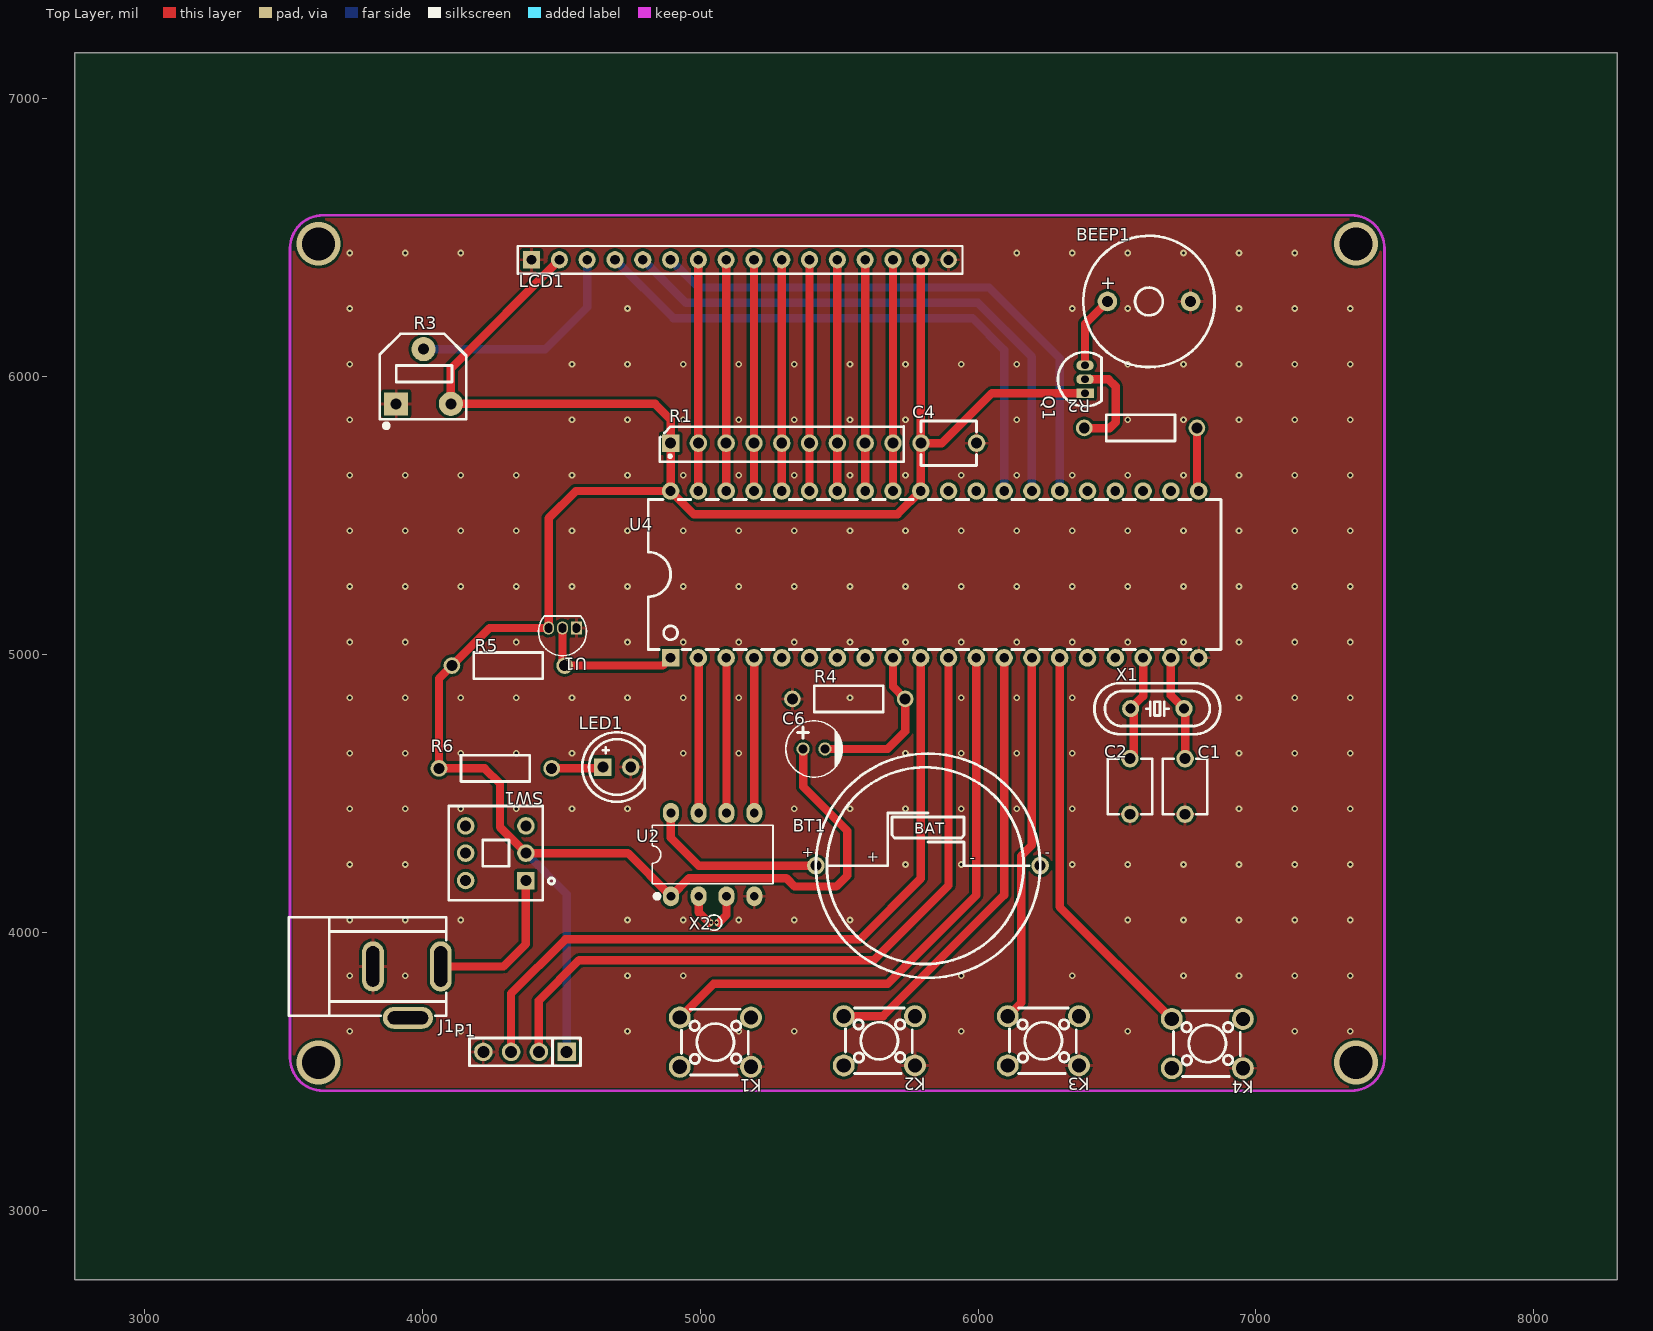
[diagram p0: Top Layer view]
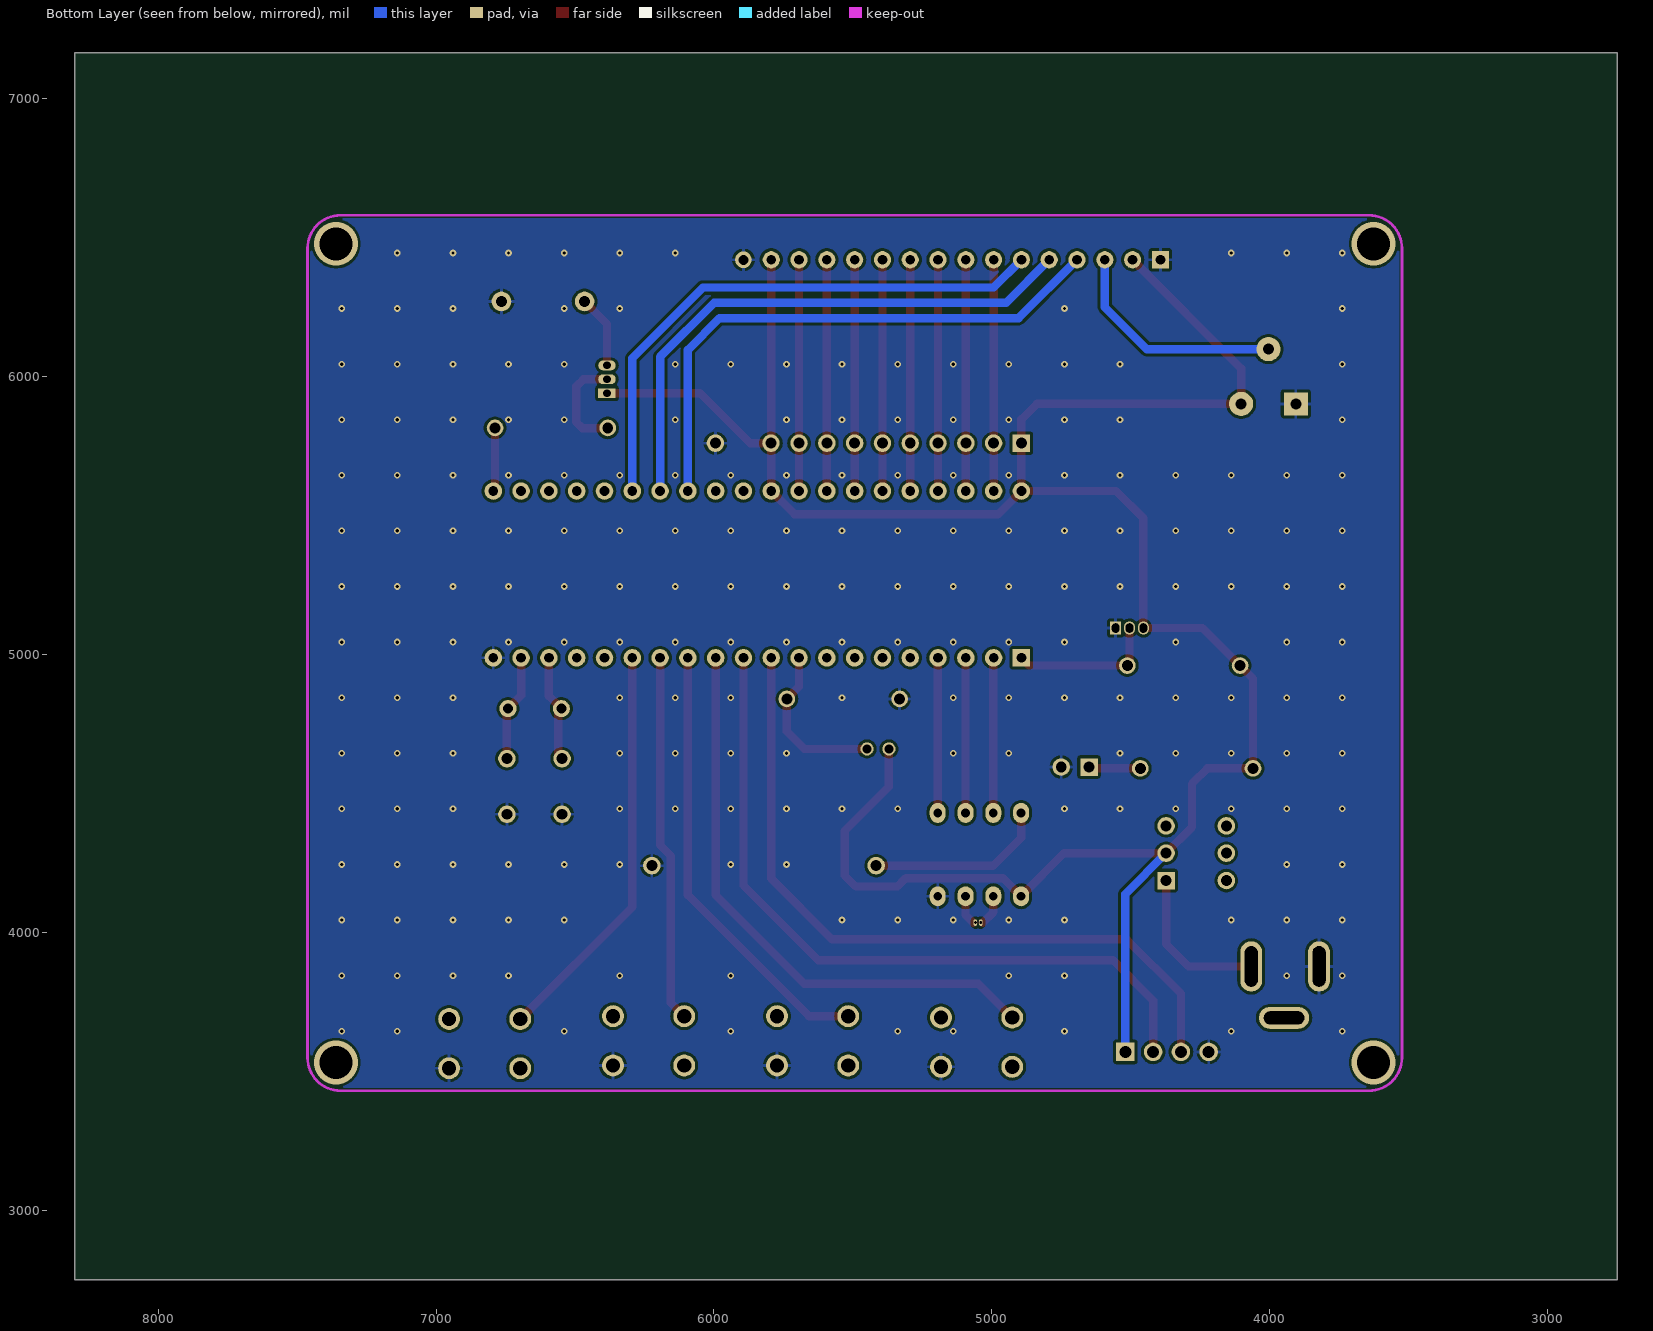
[diagram p1: Bottom Layer view, seen from below]
# Altium PCB MISC51325.pcbdoc
Units mil, origin at the board's own origin, x right, y up, seen from the top; angles counter-clockwise.
Board outline 5550 x 4415 mil, 2 copper layers (Top Layer, Bottom Layer), stack 62.206 mil thick; 27 components, 35 nets, 137 pads, 209 vias.

## Layer stack, top to bottom
Top Solder Mask Layer: solder mask 0.394, Dk 3.3
Top Layer: signal copper 1.379
Dielectric1: surface 59.449, FR4, Dk 4.5
Bottom Layer: signal copper 1.378
Bottom Solder Mask Layer: solder mask 0.394, Dk 3.3

## Board outline
8300,2750 2750,2750 2750,7165 8300,7165

## Design rules (kind name [scope] priority, off if disabled: settings)
BoardOutlineClearance copperThickness2oz_1 [All] p2 off: genericclearance=7.99 ignorepadtopadclearanceinfootprint=FALSE except(0: Arc-SplitContinuation Track-SplitContinuation SMDPad-SplitContinuation THPad-SplitContinuation Via-SplitContinuation Fill-SplitContinuation Region-SplitContinuation Poly-SplitContinuation Text-SplitContinuation Hole-SplitContinuation; 5.98: Arc-CutoutEdge SMDPad-CutoutEdge THPad-CutoutEdge Via-CutoutEdge Fill-CutoutEdge Region-CutoutEdge Text-CutoutEdge; 6.93: Hole-OutlineEdge Hole-CutoutEdge; 10: Poly-OutlineEdge Poly-CutoutEdge; 11.81: Arc-OutlineEdge Track-OutlineEdge SMDPad-OutlineEdge THPad-OutlineEdge Via-OutlineEdge Fill-OutlineEdge Region-OutlineEdge Text-OutlineEdge Track-CutoutEdge)
BoardOutlineClearance copperThickness1oz_1 [All] p4: genericclearance=4.02 ignorepadtopadclearanceinfootprint=FALSE except(0: Arc-SplitContinuation Track-SplitContinuation SMDPad-SplitContinuation THPad-SplitContinuation Via-SplitContinuation Fill-SplitContinuation Region-SplitContinuation Poly-SplitContinuation Text-SplitContinuation Hole-SplitContinuation; 6: SMDPad-CutoutEdge THPad-CutoutEdge Via-CutoutEdge Fill-CutoutEdge Region-CutoutEdge Text-CutoutEdge; 6.93: Hole-OutlineEdge Hole-CutoutEdge; 10: Poly-OutlineEdge Poly-CutoutEdge; 11.8: Arc-OutlineEdge Track-OutlineEdge SMDPad-OutlineEdge THPad-OutlineEdge Via-OutlineEdge Fill-OutlineEdge Region-OutlineEdge Text-OutlineEdge; 11.81: Arc-CutoutEdge Track-CutoutEdge)
Clearance copperThickness2oz [All] p1 off: gap=7.99 ignorepadtopadclearanceinfootprint=FALSE except(5.98: SMDPad-Track SMDPad-SMDPad THPad-Track SMDPad-THPad THPad-THPad Track-Via SMDPad-Via THPad-Via Via-Via Fill-Track Region-Track Fill-SMDPad Region-SMDPad Fill-THPad Region-THPad Fill-Via Region-Via Fill-Fill Fill-Region Region-Region Arc-Track Arc-SMDPad Arc-THPad Arc-Via Fill-Arc Region-Arc Arc-Arc Text-Track SMDPad-Text Text-THPad Text-Via Fill-Text Region-Text Arc-Text Text-Text; 6.93: Hole-Track Hole-SMDPad Hole-THPad Hole-Via Fill-Hole Region-Hole Hole-Arc Hole-Text; 10: Poly-Track Poly-SMDPad Poly-THPad Poly-Via Poly-Fill Poly-Region Poly-Poly Poly-Arc Poly-Text Poly-Hole)
Clearance copperThickness1oz [All] p3: gap=4.02 ignorepadtopadclearanceinfootprint=FALSE except(5.98: SMDPad-Track SMDPad-SMDPad THPad-Track SMDPad-THPad THPad-THPad Track-Via SMDPad-Via THPad-Via Via-Via Fill-Track Region-Track Fill-SMDPad Region-SMDPad Fill-THPad Region-THPad Fill-Via Region-Via Fill-Fill Fill-Region Region-Region; 6: Arc-Track Arc-SMDPad Arc-THPad Arc-Via Fill-Arc Region-Arc Arc-Arc Text-Track SMDPad-Text Text-THPad Text-Via Fill-Text Region-Text Arc-Text Text-Text; 6.93: Hole-Track Hole-SMDPad Hole-THPad Hole-Via Fill-Hole Region-Hole Hole-Arc Hole-Text; 10: Poly-Track Poly-SMDPad Poly-THPad Poly-Via Poly-Fill Poly-Region Poly-Poly Poly-Arc Poly-Text Poly-Hole)
DiffPairsRouting differentialPair [All] p1: maxlimit=6 minlimit=6 mostfreqgap=6 toplayer_minwidth=5 toplayer_prefwidth=10 toplayer_maxwidth=100 toplayer_mingap=6 toplayer_prefgap=6 toplayer_maxgap=6 bottomlayer_minwidth=5 bottomlayer_prefwidth=10 bottomlayer_maxwidth=100 bottomlayer_mingap=6 bottomlayer_prefgap=6 bottomlayer_maxgap=6 maxuncoupledlength=10
HoleToHoleClearance otherClearance [All] p1: gap=11.81 allowstackedmicrovias=TRUE
Length netLength [All] p1: minlimit=0 maxlimit=0
MatchedLengths netLengthTolerance [All] p1: tolerance=1000
PasteMaskExpansion pasteMaskExpansion [All] p1: expansion=0
PlaneConnect innerPlane [All] p1: planeconnectstyle=Relief reliefexpansion=20 reliefentries=4 reliefconductorwidth=10 reliefairgap=10
PolygonConnect copperRegion [(InNet('GND'))] p1: connectstyle=Relief reliefconductorwidth=10 reliefentries=4 polygonreliefangle="90 Angle" airgapwidth=10 via.connectstyle=Relief via.reliefconductorwidth=10 via.reliefentries=4 via.polygonreliefangle="90 Angle" via.airgapwidth=10
RoutingVias viaSize [All] p1: holewidth=12.01 width=24.02 viastyle="Through Hole" minholewidth=11.81 minwidth=19.68 maxholewidth=248.03 maxwidth=393.7
SolderMaskExpansion solderMaskExpansion [IsVia] p1: expansion=-1000 istentingtop=TRUE
SolderMaskExpansion solderMaskExpansion [All] p2: expansion=2 istentingtop=FALSE
Width copperThickness2oz_2 [All] p1 off: maxlimit=100 minlimit=8 preferedwidth=10
Width copperThickness1oz_2 [All] p2: maxlimit=100 minlimit=5 preferedwidth=10

## Components (designator, comment, footprint, x,y, rotation, side; value= is the part's Value field where it differs from the comment)
BEEP1 "" BUZ-TH_BD12.0-P7.60-D0.6-FD 6615,6270 r0 top
BT1 "Battery" BAT-TH_CR2032 5820,4240 r0 top
C1 "30pF" CAP-TH_L5.0-W4.0-P5.00-D1.0 6745,4525 r90 top
C2 "30pF" CAP-TH_L5.0-W4.0-P5.00-D1.0 6546.5,4525 r90 top
C4 "0.1uF" CAP-TH_L5.0-W4.0-P5.00-D1.0 5895,5760 r0 top
C6 "10uF" CAP-TH_BD5.0-P2.00-D0.6-FD 5410,4660 r0 top
J1 "" DC-005_2.5 3940,3865 r180 top
K1 "" KEY-TH_4P-L6.0-W6.0-P4.50-LS6.50 5055,3605 r180 top
K2 "" KEY-TH_4P-L6.0-W6.0-P4.50-LS6.50 5645,3610 r180 top
K3 "" KEY-TH_4P-L6.0-W6.0-P4.50-LS6.50 6235,3610 r180 top
K4 "" KEY-TH_4P-L6.0-W6.0-P4.50-LS6.50 6825,3600 r180 top
LCD1 "1602" HDR-M-2.54_1X16 5143.88,6420 r0 top
LED1 "" LED-TH_5mm 4700.63,4595 r0 top
P1 "" HDR-TH_4P-P2.54-V-M 4370,3570 r180 top
Q1 "8550" S8550P_TO-92 6385,5990 r90 top
R1 "" SIP-9_L22.3-W3.2-P2.54_KA2284-SIP-9 5293.88,5760 r0 top
R2 "1K" Res_1/4W 6585,5815 r0 top
R3 "103" RES-ADJ-SMD_RM065-V1 4005,6000 r0 top
R4 "10K" Res_1/4W 5535,4840 r0 top
R5 "4.7K" Res_1/4W 4310,4960 r180 top
R6 "1K" Res_1/4W 4263.44,4590 r0 top
SW1 "SWT" SW-TH_6P-L8.5-W8.5-P2.50-LS5.5-BL-2 4265,4285 r90 top
U1 "DS18B20" TO-92-3_L4.5-W3.5-P1.27-L 4505,5095 r180 top
U2 "DS1302" DIP-8_L10.9-W6.4-P2.54-LS7.6-BL 5045,4280 r0 top
U4 "STC89C52RC-40I-PDIP40" DIP-40_L52.0-W13.7-P2.54-LS15.2-BL 5843.88,5287.97 r0 top
X1 "12M" HC-49S_L11.5-W4.7-P4.88 6645,4805 r0 top
X2 "32.768kHz" CRYSTAL-TH_BD1.4-P0.45-D0.2 5050,4035 r180 top

## Footprints (in the part's own frame and the unit in brackets; to place one, negate y for a bottom-side part, rotate by r counter-clockwise, add the part's x,y. Pads: shape width x height; smd on the part's side, far side on the other; paste and mask are expansions set on the pad)
BAT-TH_CR2032 [mm]
  round 1.6 hole 1: 1(-10.25,0) 2(10.25,0)
  silkscreen extent -10.25,-10.25 10.25,10.25
BUZ-TH_BD12.0-P7.60-D0.6-FD [mm]
  round 1.8 hole 1: 1(-3.8,0) 2(3.8,0)
  silkscreen extent -6,-6 6,6
CAP-TH_BD5.0-P2.00-D0.6-FD [mm]
  round 1.201 hole 0.801: 1(-1,0) 2(1,0)
  silkscreen extent -2.58,-2.57 2.59,2.57
CAP-TH_L5.0-W4.0-P5.00-D1.0 [mm]
  round 1.6 hole 1: 1(-2.54,0) 2(2.54,0)
  silkscreen extent -2.54,-2.03 2.54,2.03
CRYSTAL-TH_BD1.4-P0.45-D0.2 [mm]
  oval 0.32x0.6 hole 0.27 paste+0 mask+0.05: 1(-0.25,0) 2(0.25,0)
  silkscreen extent -0.7,-0.7 0.7,0.7
DC-005_2.5 [mm]
  oval 2x4.6 hole 1.2 slot 3.7 at 90 deg paste+0 mask+0.051: 1(-3.227,-0.318) 2(2.973,-0.318)
  oval 4.6x2 hole 1.2 slot 3.7 at 0 deg paste+0 mask+0.051: 3(-0.227,4.382)
  silkscreen extent -3.73,-4.82 10.67,4.18
DIP-8_L10.9-W6.4-P2.54-LS7.6-BL [mm]
  oval 1.462x1.828 hole 0.8: 1(-3.81,-3.81) 2(-1.27,-3.81) 3(1.27,-3.81) 4(3.81,-3.81) 5(3.81,3.81) 6(1.27,3.81) 7(-1.27,3.81) 8(-3.81,3.81)
  silkscreen extent -5.53,-4.01 5.53,2.67
DIP-40_L52.0-W13.7-P2.54-LS15.2-BL [mil]
  rect 63x63 hole 35: 1(-950,-300)
  round 63 hole 35: 2(-850,-300) 3(-750,-300) 4(-650,-300) 5(-550,-300) 6(-450,-300) 7(-350,-300) 8(-250,-300) 9(-150,-300) 10(-50,-300) 11(50,-300) 12(150,-300) 13(250,-300) 14(350,-300) 15(450,-300) 16(550,-300) 17(650,-300) 18(750,-300) 19(850,-300) 20(950,-300) 21(950,300) 22(850,300) 23(750,300) 24(650,300) 25(550,300) 26(450,300) 27(350,300) 28(250,300) 29(150,300) 30(50,300) 31(-50,300) 32(-150,300) 33(-250,300) 34(-350,300) 35(-450,300) 36(-550,300) 37(-650,300) 38(-750,300) 39(-850,300) 40(-950,300)
  silkscreen extent -1030,-270 1030,270
HC-49S_L11.5-W4.7-P4.88 [mm]
  round 1.56 hole 0.9: 1(-2.44,0) 2(2.44,0)
  silkscreen extent -5.75,-2.33 5.75,2.33
HDR-M-2.54_1X16 [mil]
  rect 62x62 hole 35: 1(-750,0)
  round 62 hole 35: 2(-650,0) 3(-550,0) 4(-450,0) 5(-350,0) 6(-250,0) 7(-150,0) 8(-50,0) 9(50,0) 10(150,0) 11(250,0) 12(350,0) 13(450,0) 14(550,0) 15(650,0)
  round 60 hole 36: 16(750,0)
  silkscreen extent -800,-50 800,50
HDR-TH_4P-P2.54-V-M [mm]
  rect 1.7x1.7 hole 1.1: 1(-3.81,0)
  round 1.7 hole 1.1: 2(-1.27,0) 3(1.27,0) 4(3.81,0)
  silkscreen extent -5.08,-1.27 5.08,1.27
KEY-TH_4P-L6.0-W6.0-P4.50-LS6.50 [mm]
  round 2 hole 1.3: 1(-3.25,2.25) 2(3.25,2.25) 3(-3.25,-2.25) 4(3.25,-2.25)
  silkscreen extent -3,-3 3.1,3
LED-TH_5mm [mm]
  rect 1.6x1.6 hole 1 paste+0 mask+0.051: 1(-1.27,0)
  round 1.6 hole 1 paste+0 mask+0.051: 2(1.27,0)
  silkscreen extent -3.17,-3.17 2.54,3.17
RES-ADJ-SMD_RM065-V1 [mm]
  rect 2.2x2.1 hole 1 paste+0 mask+0.05: 1(-2.5,-2.5)
  round 2.2 hole 1 paste+0 mask+0.05: 2(0,2.5) 3(2.5,-2.5)
  silkscreen extent -4,-4.7 3.9,3.9
Res_1/4W [mil]
  round 60 hole 39.37 paste+0 mask+2: 1(-202.76,0) 2(202.76,0)
  silkscreen extent -124,-47 124,47
S8550P_TO-92 [mm]
  rect 0.9x1.6 hole 0.7 paste+0 mask+0.051: 1(-1.27,0)
  oval 0.9x1.6 hole 0.7 paste+0 mask+0.051: 2(0,0) 3(1.27,0)
  silkscreen extent -2.48,-1.5 2.48,2.48
SIP-9_L22.3-W3.2-P2.54_KA2284-SIP-9 [mm]
  rect 1.6x1.6 hole 1: 1(-10.16,0)
  round 1.6 hole 1: 2(-7.62,0) 3(-5.08,0) 4(-2.54,0) 5(0,0) 6(2.54,0) 7(5.08,0) 8(7.62,0) 9(10.16,0)
  silkscreen extent -11.15,-1.69 11.15,1.52
SW-TH_6P-L8.5-W8.5-P2.50-LS5.5-BL-2 [mm]
  rect 1.6x1.6 hole 1: 1(-2.5,-2.75)
  round 1.6 hole 1: 2(0,-2.75) 3(2.5,-2.75) 4(2.5,2.75) 5(0,2.75) 6(-2.5,2.75)
  silkscreen extent -4.3,-5.36 4.3,4.3
TO-92-3_L4.5-W3.5-P1.27-L [mm]
  rect 1x1.2 hole 0.7 slot 0.85 at 90 deg: 1(-1.27,0)
  oval 1x1.2 hole 0.7 slot 0.85 at 90 deg: 2(0,0) 3(1.27,0)
  silkscreen extent -2.19,-1.1 2.19,2.52

## Via types
v1: diameter 24.02, hole 12, Top Layer to Bottom Layer, 205 vias
v2: diameter 157.48, hole 118.1, Top Layer to Bottom Layer, 4 vias

## Nets (pads, with @x,y where several pads share a name; then routed paths per layer and width w, separated by ;. In a path a pad name is that pad's centre, name@x,y a point inside that pad or via, vN(x,y) a via of type N, cw(c..) or ccw(c..) an arc to the next point about the centre after c; other vN are vias at no path point)
$2N34: J1.1 SW1.1 | length 568
  Top Layer w30: J1.1 4292.52,3877.51 4373.27,3958.27 SW1.1
$2N37: BEEP1.1 Q1.3 | length 263.3
  Top Layer w30: Q1.3 6385,6189.6 BEEP1.1
$2N47: U2.2 X2.2 | length 110.6
  Top Layer w30: U2.2 4995,4072.56 5032.56,4035
$2N48: U2.3 X2.1 | length 106.4
  Top Layer w30: 5067.44,4035 5095,4062.56 U2.3
$2N51: BT1.1 U2.8 | length 652.9
  Top Layer w30: U2.8 4895,4340 4995,4240 BT1.1
$2N72: C6.2 R4.2 U4.9 | length 597.8
  Top Layer w30: C6.2 5675,4660 5737.76,4722.76 R4.2 5693.88,4883.88 U4.9
$2N199: LCD1.3 R3.2 | length 822.3
  Bottom Layer w30: R3.2 4443.43,6098.43 4593.88,6248.88 LCD1.3
$2N200: Q1.2 R2.1 | length 372.4
  Top Layer w30: R2.1 6383.45,5813.79 6473.79,5813.79 6495,5835 6495,5965 6470,5990 Q1.2
$2N202: LED1.1 R6.2 | length 186.5
  Top Layer w30: R6.2 4645.63,4590 LED1.1
BEEP: R2.2 U4.21 | length 229.6
  Top Layer w30: R2.2 6787.76,5594.09 U4.21
D0: LCD1.7 R1.2 U4.39 | length 832
  Top Layer w30: U4.39 R1.2 LCD1.7
D1: LCD1.8 R1.3 U4.38 | length 832
  Top Layer w30: U4.38 R1.3 LCD1.8
D2: LCD1.9 R1.4 U4.37 | length 832
  Top Layer w30: U4.37 R1.4 LCD1.9
D3: LCD1.10 R1.5 U4.36 | length 832
  Top Layer w30: U4.36 R1.5 LCD1.10
D4: LCD1.11 R1.6 U4.35 | length 832
  Top Layer w30: U4.35 R1.6 LCD1.11
D5: LCD1.12 R1.7 U4.34 | length 832
  Top Layer w30: U4.34 R1.7 LCD1.12
D6: LCD1.13 R1.8 U4.33 | length 832
  Top Layer w30: U4.33 R1.8 LCD1.13
D7: LCD1.14 R1.9 U4.32 | length 832
  Top Layer w30: U4.32 R1.9 LCD1.14
DQ: R5.1 U1.2 U4.1 | length 530.9
  Top Layer w30: U1.2 4505,4967.76 R5.1 4865.91,4960 U4.1
EN: LCD1.6 U4.26 | length 2024.7
  Bottom Layer w30: LCD1.6 4993.88,6320 6040,6320 6293.88,6066.12 U4.26
GND: BEEP1.2 BT1.2 C1.1 C2.1 C4.2 J1.2 K1.1 K2.1 K3.1 K4.1 LCD1.1 LCD1.16 LED1.2 P1.4 R3.1 R4.1 U1.1 U2.4 U4.20
  other v1: 3739.1,3644.49 4139.1,3644.49 4739.1,3644.49 5139.1,3644.49 5339.1,3644.49 5939.1,3644.49 6539.1,3644.49 7139.1,3644.49 7339.1,3644.49 3739.1,3844.49 3939.1,3844.49 4739.1,3844.49 4939.1,3844.49 5939.1,3844.49 6339.1,3844.49 6739.1,3844.49 6939.1,3844.49 7139.1,3844.49 7339.1,3844.49 3739.1,4044.49 3939.1,4044.49 4139.1,4044.49 4739.1,4044.49 4939.1,4044.49 5139.1,4044.49 5339.1,4044.49 5539.1,4044.49 6539.1,4044.49 6739.1,4044.49 6939.1,4044.49 7139.1,4044.49 7339.1,4044.49 3739.1,4244.49 3939.1,4244.49 5739.1,4244.49 5939.1,4244.49 6339.1,4244.49 6539.1,4244.49 6739.1,4244.49 6939.1,4244.49 7139.1,4244.49 7339.1,4244.49 3739.1,4444.49 3939.1,4444.49 4139.1,4444.49 4339.1,4444.49 4539.1,4444.49 4739.1,4444.49 5339.1,4444.49 5539.1,4444.49 5739.1,4444.49 5939.1,4444.49 6139.1,4444.49 6339.1,4444.49 6939.1,4444.49 7139.1,4444.49 7339.1,4444.49 3739.1,4644.49 3939.1,4644.49 4139.1,4644.49 4339.1,4644.49 4539.1,4644.49 4939.1,4644.49 5139.1,4644.49 5739.1,4644.49 5939.1,4644.49 6139.1,4644.49 6339.1,4644.49 6939.1,4644.49 7139.1,4644.49 7339.1,4644.49 3739.1,4844.49 3939.1,4844.49 4139.1,4844.49 4339.1,4844.49 4539.1,4844.49 4739.1,4844.49 4939.1,4844.49 5139.1,4844.49 5539.1,4844.49 5939.1,4844.49 6139.1,4844.49 6339.1,4844.49 6939.1,4844.49 7139.1,4844.49 7339.1,4844.49 3739.1,5044.49 3939.1,5044.49 4339.1,5044.49 4739.1,5044.49 4939.1,5044.49 5139.1,5044.49 5339.1,5044.49 5539.1,5044.49 5739.1,5044.49 5939.1,5044.49 6139.1,5044.49 6339.1,5044.49 6539.1,5044.49 6739.1,5044.49 6939.1,5044.49 7139.1,5044.49 7339.1,5044.49 3739.1,5244.49 3939.1,5244.49 4139.1,5244.49 4339.1,5244.49 4539.1,5244.49 4739.1,5244.49 4939.1,5244.49 5139.1,5244.49 5339.1,5244.49 5539.1,5244.49 5739.1,5244.49 5939.1,5244.49 6139.1,5244.49 6339.1,5244.49 6539.1,5244.49 6739.1,5244.49 6939.1,5244.49 7139.1,5244.49 7339.1,5244.49 3739.1,5444.49 3939.1,5444.49 4139.1,5444.49 4339.1,5444.49 4539.1,5444.49 4739.1,5444.49 4939.1,5444.49 5139.1,5444.49 5339.1,5444.49 5539.1,5444.49 5739.1,5444.49 5939.1,5444.49 6139.1,5444.49 6339.1,5444.49 6539.1,5444.49 6739.1,5444.49 6939.1,5444.49 7139.1,5444.49 7339.1,5444.49 3739.1,5644.49 3939.1,5644.49 4139.1,5644.49 4339.1,5644.49 4539.1,5644.49 4739.1,5644.49 4939.1,5644.49 5139.1,5644.49 5339.1,5644.49 5539.1,5644.49 5739.1,5644.49 5939.1,5644.49 6139.1,5644.49 6339.1,5644.49 6539.1,5644.49 6739.1,5644.49 6939.1,5644.49 7139.1,5644.49 7339.1,5644.49 3739.1,5844.49 4539.1,5844.49 4739.1,5844.49 4939.1,5844.49 5139.1,5844.49 5339.1,5844.49 5539.1,5844.49 5739.1,5844.49 6139.1,5844.49 6539.1,5844.49 6739.1,5844.49 6939.1,5844.49 7139.1,5844.49 7339.1,5844.49 3739.1,6044.49 4539.1,6044.49 4739.1,6044.49 4939.1,6044.49 5139.1,6044.49 5339.1,6044.49 5539.1,6044.49 5739.1,6044.49 5939.1,6044.49 6139.1,6044.49 6539.1,6044.49 6739.1,6044.49 6939.1,6044.49 7139.1,6044.49 7339.1,6044.49 3739.1,6244.49 4739.1,6244.49 6339.1,6244.49 6539.1,6244.49 6939.1,6244.49 7139.1,6244.49 7339.1,6244.49 3739.1,6444.49 3939.1,6444.49 4139.1,6444.49 6139.1,6444.49 6339.1,6444.49 6539.1,6444.49 6739.1,6444.49 6939.1,6444.49 7139.1,6444.49
IO: U2.6 U4.3 | length 558.4
  Top Layer w30: U4.3 5095,4986.85 U2.6
KEY1: K1.4 U4.12 | length 2103.3
  Top Layer w30: K1.4 5048.47,3815 5675,3815 5993.88,4133.88 U4.12
KEY2: K2.4 U4.13 | length 1611.2
  Top Layer w30: K2.4 5658.58,3698.58 6093.88,4133.88 U4.13
KEY3: K3.4 U4.14 | length 1325.4
  Top Layer w30: K3.4 6155,3746.53 6155,4275 6193.88,4313.88 U4.14
KEY4: K4.4 U4.15 | length 1466.4
  Top Layer w30: U4.15 6293.88,4091.75 K4.4
P3.0: P1.3 U4.10 | length 2649.4
  Top Layer w30: P1.3 4320,3780 4515,3975 5575,3975 5793.88,4193.88 U4.10
P3.1: P1.2 U4.11 | length 2649.4
  Top Layer w30: P1.2 4420,3755 4565,3900 5625,3900 5893.88,4168.88 U4.11
RS: LCD1.4 U4.28 | length 2042.3
  Bottom Layer w30: LCD1.4 4903.88,6210 5980,6210 6093.88,6096.12 U4.28
RST: U2.5 U4.4 | length 558.4
  Top Layer w30: U4.4 5195,4986.85 U2.5
RW: LCD1.5 U4.27 | length 2027.7
  Bottom Layer w30: LCD1.5 4948.88,6265 6000,6265 6193.88,6071.12 U4.27
SCLK: U2.7 U4.2 | length 558.4
  Top Layer w30: U4.2 4995,4986.85 U2.7
VCC: C4.1 C6.1 LCD1.2 LCD1.15 P1.1 Q1.1 R1.1 R3.3 R5.2 R6.1 SW1.2 U1.3 U2.1 U4.31 U4.40 | length 8988.9
  Top Layer w30: LCD1.2 4103.43,6029.55 R3.3 4838.43,5901.57 4893.88,5846.12 R1.1 U4.40 ; C6.1 5370.63,4524.37 5530,4365 5530,4205 5490,4165 5340,4165 5310,4195 4960,4195 U2.1 4740.01,4284.99 SW1.2 4280,4378.27 4280,4535 4225,4590 R6.1 4060.68,4913.44 R5.2 4242.24,5095 U1.3 4455,5490 4552.97,5587.97 U4.40 ; LCD1.15 U4.31 5710.91,5505 4976.85,5505 U4.40 ; C4.1 5870,5760 6050,5940 Q1.1
  Bottom Layer w30: SW1.2 4520,4138.27 P1.1
XTAL1: C1.2 U4.19 X1.2 | length 384.1
  Top Layer w30: U4.19 6693.88,4852.18 X1.2 6745,4801.06 C1.2
XTAL2: C2.2 U4.18 X1.1 | length 391.8
  Top Layer w30: C2.2 6560,4638.51 6560,4793.94 X1.1 6593.88,4849.94 U4.18
pads on no net: J1.3 K1.2 K1.3 K2.2 K2.3 K3.2 K3.3 K4.2 K4.3 SW1.3 SW1.4 SW1.5 SW1.6 U4.5 U4.6 U4.7 U4.8 U4.16 U4.17 U4.22 U4.23 U4.24 U4.25 U4.29 U4.30
copper on no net:
  other v2: 3627.36,3532.36 7359.65,3532.36 3627.36,6477.24 7359.65,6477.24

## Polygon pours and split planes (outlines as drawn)
GND on Bottom Layer (solid, remove dead copper, pour order 2): 3000,6915 3000,3000 8050,3000 8050,6915
GND on Top Layer (solid, remove dead copper, pour order 0): 3290,6780 3290,3240 7985,3240 7985,6780

## Keep-outs
Board Outline Layer:
  lines w10: 3525,3548.5 3525,6461.89 cw(c3643.11,6461.89) 3643.11,6580 7343.9,6580 cw(c7343.9,6461.89) 7462.01,6461.89 7462.01,3548.5 cw(c7343.9,3548.5) 7343.9,3430.39 3643.11,3430.39 cw(c3643.11,3548.5) 3525,3548.5